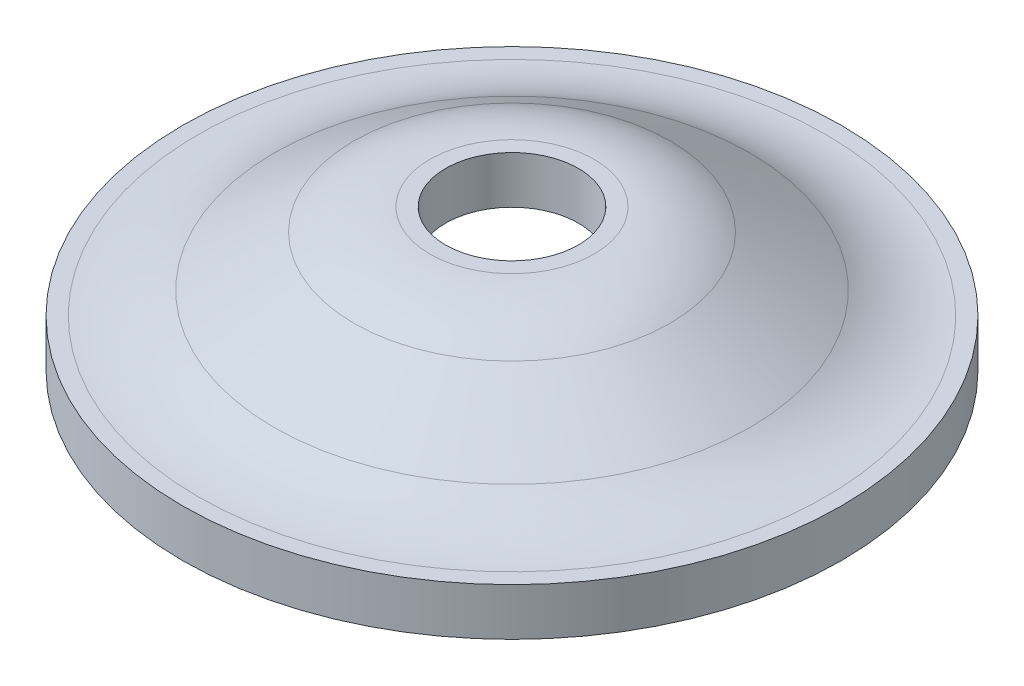
from build123d import *


with BuildPart() as part:
    # Sketch1 → Revolve1 (revolve)
    with BuildSketch(Plane.XY, mode=Mode.PRIVATE) as revolve1_sk:
        with BuildLine():
            Line((-2.8, 0), (-3.463509174, 0))
            ThreePointArc((-3.463509174, 0), (-5.131546288, -0.236524296), (-6.668072967, -0.927449272))
            Line((-6.668072967, -0.927449272), (-10.031927033, -3.052550728))
            ThreePointArc((-10.031927033, -3.052550728), (-11.568453712, -3.743475704), (-13.236490826, -3.98))
            Line((-13.236490826, -3.98), (-13.9, -3.98))
            Line((-13.9, -3.98), (-13.9, -5.98))
            Line((-13.9, -5.98), (-13.236490826, -5.98))
            ThreePointArc((-13.236490826, -5.98), (-11.568453712, -5.743475704), (-10.031927033, -5.052550728))
            Line((-10.031927033, -5.052550728), (-6.668072967, -2.927449272))
            ThreePointArc((-6.668072967, -2.927449272), (-5.131546288, -2.236524296), (-3.463509174, -2))
            Line((-3.463509174, -2), (-2.8, -2))
            Line((-2.8, -2), (-2.8, 0))
        make_face()
    revolve(revolve1_sk.sketch.rotate(Axis((0, 0, 0), (0, -1, 0)), 270), axis=Axis((0, 0, 0), (0, -1, 0)))


solid = part.part
